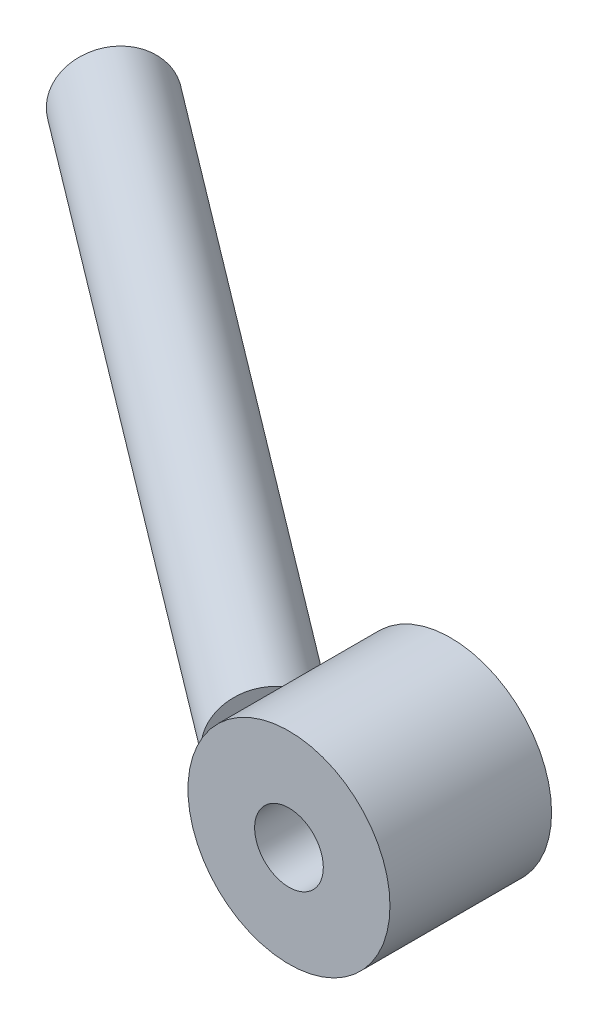
from build123d import *

# Parameters (mm, degrees)
SKETCH1_R           = 12.5
BOSS_EXTRUDE1_DEPTH = 10
M10_TAPPED_HOLE1_D  = 8.5
CHAMFER1_SIZE       = 2


with BuildPart() as part:
    # Sketch1 → Boss-Extrude1 (new, symmetric)
    with BuildSketch(Plane.XY):
        Circle(SKETCH1_R)
    extrude(amount=BOSS_EXTRUDE1_DEPTH, both=True)

    # M10 Tapped Hole1 (through all)
    with Locations(Plane.XY.offset(10)):
        with Locations((0, 0)):
            Hole(M10_TAPPED_HOLE1_D / 2)

    # Sketch5 → Revolve1 (revolve)
    with BuildSketch(Plane(origin=(0, 0, 0), x_dir=(1, 0, 0), z_dir=(0, 1, 0))):
        Polygon((-12.5, 0), (-92.29474156, 60.272707085), (-88.678379135, 65.060391578), (-8.883637575, 4.787684494), align=None)
    revolve(axis=Axis((-12.5, 0, 0), (-0.7979474156035873, 0, -0.6027270708467937)))

    # Chamfer1
    chamfer1_edges = [part.edges().sort_by_distance(p)[0] for p in [
        (-95.911103985, 0, -55.485022591),
    ]]
    chamfer(chamfer1_edges, length=CHAMFER1_SIZE)


solid = part.part
